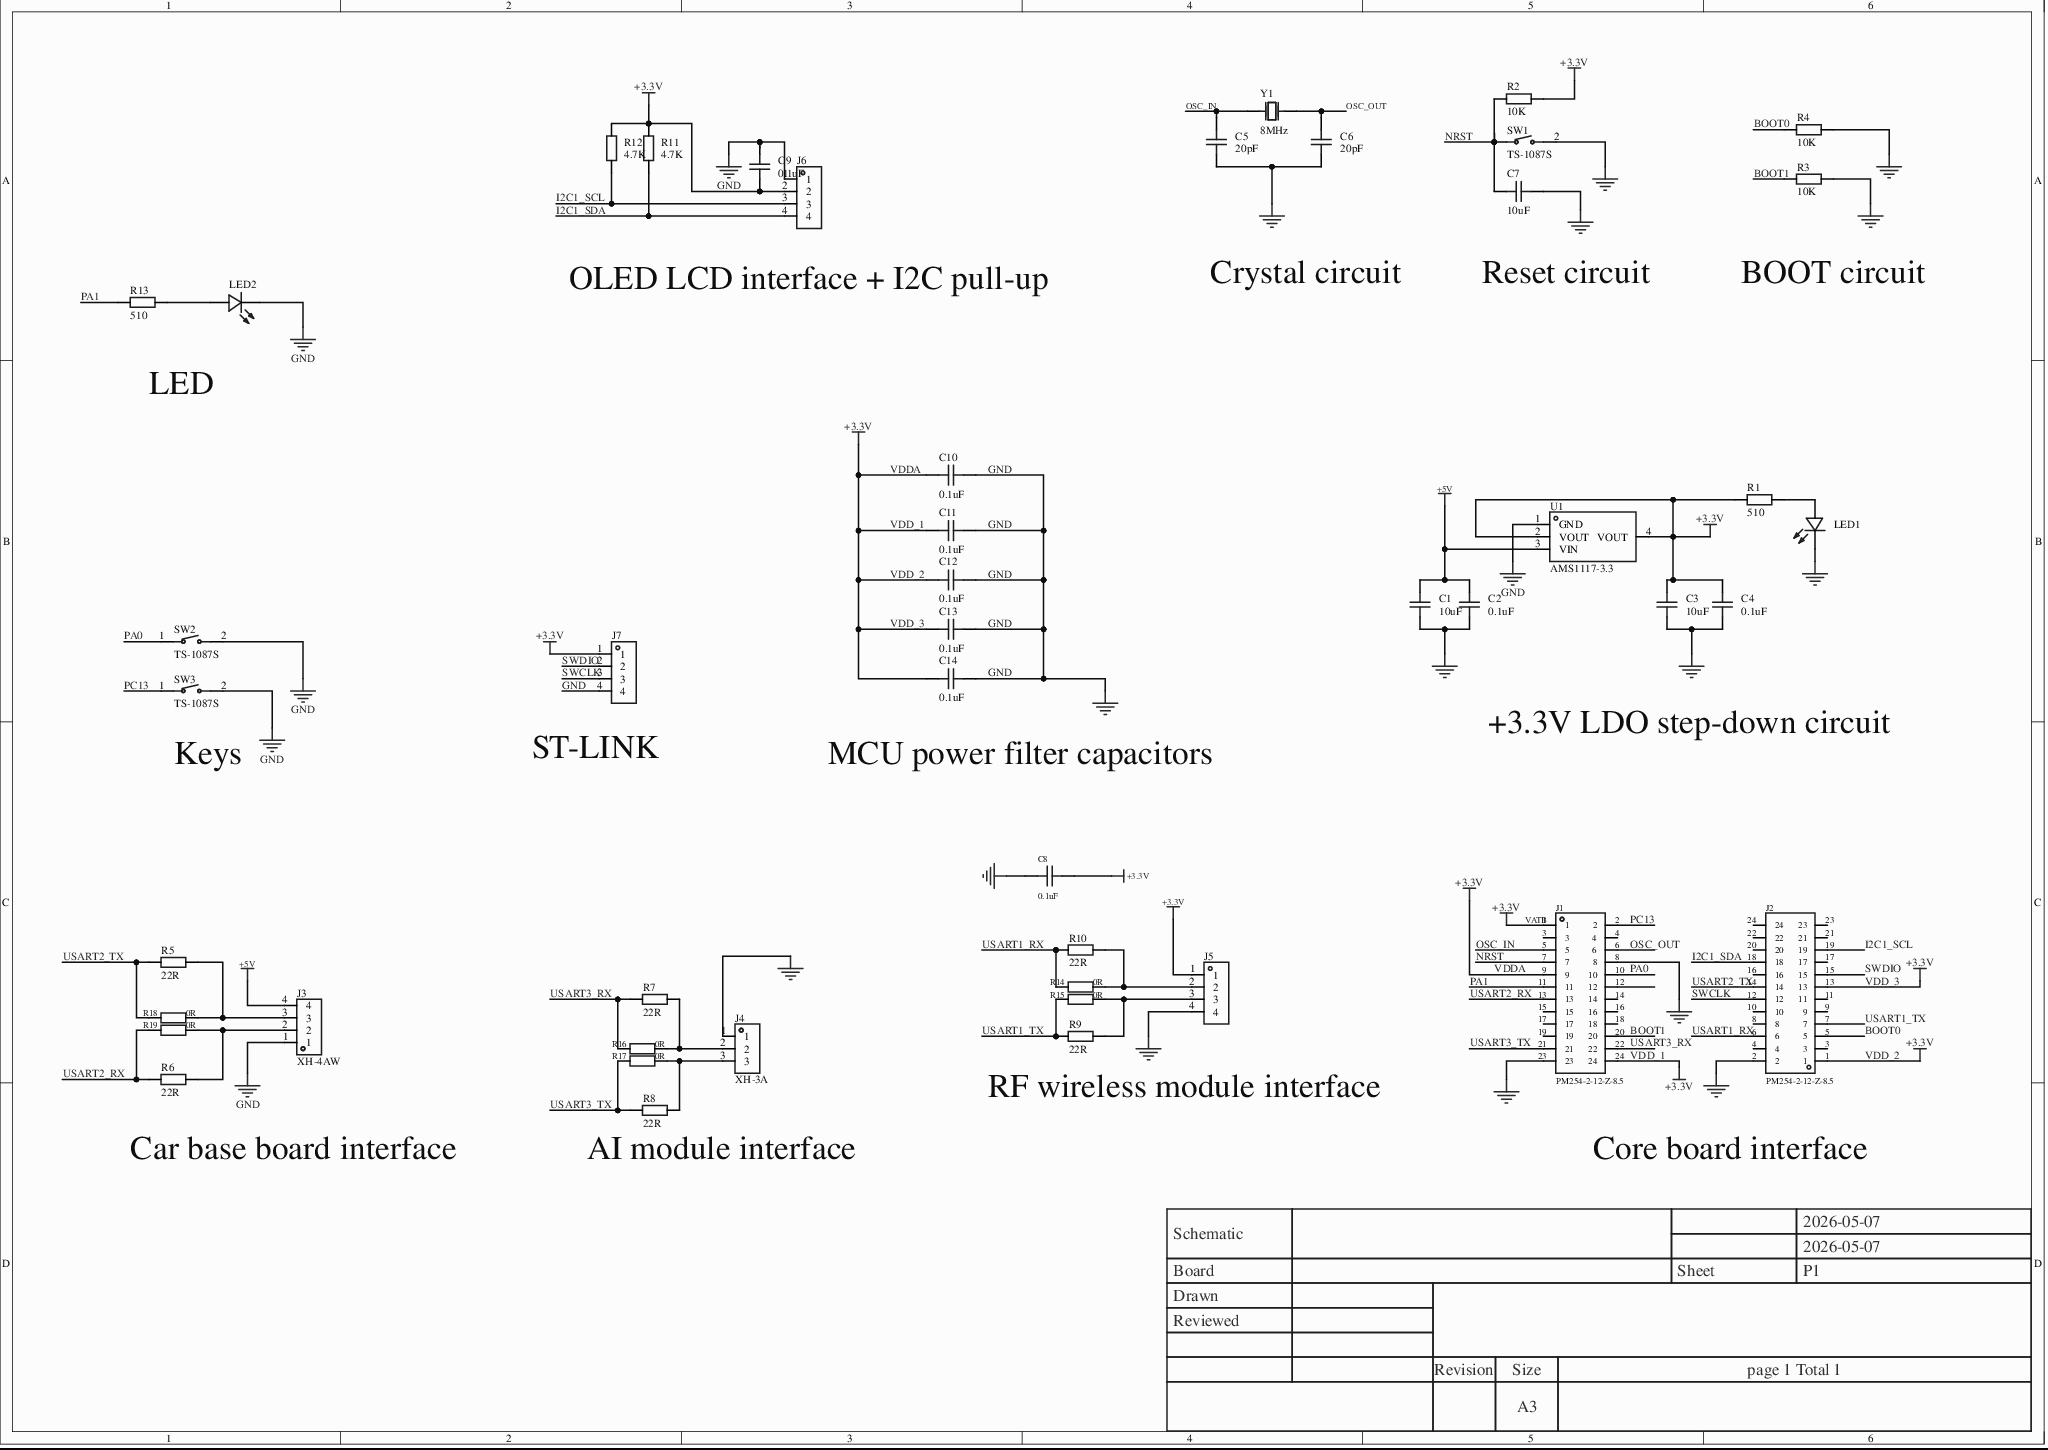
[diagram p0: MISC52078-3.schdoc]
# Altium project MISC52078-2.PrjPcb
1 sheet, 47 parts. Net scope: global (net labels, ports and power ports of the same name join across sheets).
Board file: MISC52078.pcbdoc

## Sheet MISC52078-3.schdoc
size 420 x 297 mm; Version: V1.0; @Project Name: MISC52078; @Update Date: 2026-05-23; @Create Date: 2026-05-23; @Board Name: MISC52078; @Create Time: 04:19:49; @Page Count: 1; @Page No: 1; @Schematic Name: MISC52078; @Update Time: 12:19:49; Size: A4

### Parts
C1  10uF  [C0805]
C2  0.1uF  [C0805]
C3  10uF  [C0805]
C4  0.1uF  [C0805]
C5  20pF  [C0805]
C6  20pF  [C0805]
C7  10uF  [C0805]
C8  0.1uF  [C0603]
C9  0.1uF  [C0805]
C10  0.1uF  [C0805]
C11  0.1uF  [C0805]
C12  0.1uF  [C0805]
C13  0.1uF  [C0805]
C14  0.1uF  [C0805]
J1  PM254-2-12-Z-8.5  [HDR-TH_24P-P2.54-V-F-R2-C12-S2.54-2]
J2  PM254-2-12-Z-8.5  [HDR-TH_24P-P2.54-V-F-R2-C12-S2.54-2]
J3  XH-4AW  [CONN-TH_XH-4AW]
J4  XH-3A  [CONN-TH_XH-3A]
J5  (no value)  [CONN-TH_4P-P2.54-L10.2-W2.5]
J6  (no value)  [CONN-TH_4P-P2.54-L10.2-W2.5]
J7  (no value)  [CONN-TH_4P-P2.54-L10.2-W2.5]
LED1  KT-0805W  [LED0805-R-RD]  (value not drawn)
LED2  (no value)  [LED0805-R-RD]
R1  510  [R0805]
R2  10K  [R0805]
R3  10K  [R0805]
R4  10K  [R0805]
R5  22R  [R0805]
R6  22R  [R0805]
R7  22R  [R0805]
R8  22R  [R0805]
R9  22R  [R0805]
R10  22R  [R0805]
R11  4.7K  [R0805]
R12  4.7K  [R0805]
R13  510  [R0805]
R14  0R  [R0603]
R15  0R  [R0603]
R16  0R  [R0603]
R17  0R  [R0603]
R18  0R  [R0603]
R19  0R  [R0603]
SW1  TS-1087S  [SW-SMD_L5.2-W5.2-P3.70-LS6.4]
SW2  TS-1087S  [SW-SMD_L5.2-W5.2-P3.70-LS6.4]
SW3  TS-1087S  [SW-SMD_L5.2-W5.2-P3.70-LS6.4]
U1  AMS1117-3.3  [SOT-223-3_L6.5-W3.4-P2.30-LS7.0-BR]
Y1  8MHz  [CRYSTAL-SMD_L11.5-W4.8-LS12.7]

### Nets
+5V: C1.1 C2.1 J3.4 U1.3(VIN)
GND: C1.2 C2.2 C3.1 C4.1 C5.1 C6.1 C7.2 C8.1 C9.2 C10.2 C11.2 C12.2 C13.2 C14.2 J1.8 J1.23 J2.2 J3.1 J4.1 J5.4 J6.1 J7.4 LED1.2(K) LED2.2(K) R3.2 R4.2 SW1.2 SW2.2 SW3.2 U1.1(GND)
+3.3V: C3.2 C4.2 C8.2 C9.1 C10.1 C11.1 C12.1 C13.1 C14.1 J1.1 J1.9 J1.24 J2.1 J2.13 J5.1 J6.2 J7.1 R1.1 R2.2 R11.2 R12.2 U1.2(VOUT) U1.4(VOUT)  [also labelled VATB, VDD_1, VDD_2, VDD_3, VDDA]
BOOT0: J2.5 R4.1
BOOT1: J1.20 R3.1
I2C1_SCL: J2.19 J6.3 R12.1
I2C1_SDA: J2.18 J6.4 R11.1
NRST: C7.1 J1.7 R2.1 SW1.1
OSC_IN: C5.2 J1.5 Y1.2(OSC2)
OSC_OUT: C6.2 J1.6 Y1.1(OSC1)
PA0: J1.10 SW2.1
PA1: J1.11 R13.1
PC13: J1.2 SW3.1
SWCLK: J2.12 J7.3
SWDIO: J2.15 J7.2
USART1_RX: J2.6 R10.1 R14.1
USART1_TX: J2.7 R9.1 R15.1
USART2_RX: J1.13 R6.1 R19.1
USART2_TX: J2.14 R5.1 R18.1
USART3_RX: J1.22 R7.1 R16.1
USART3_TX: J1.21 R8.1 R17.1
NetJ3_2: J3.2 R6.2 R19.2
NetJ3_3: J3.3 R5.2 R18.2
NetJ4_2: J4.2 R7.2 R16.2
NetJ4_3: J4.3 R8.2 R17.2
NetJ5_2: J5.2 R10.2 R14.2
NetJ5_3: J5.3 R9.2 R15.2
NetLED1_1: LED1.1(A) R1.2
NetLED2_1: LED2.1(A) R13.2

Not connected (* = marked no-connect by the designer): J1 3* 4* 12 14* 15* 16* 17* 18* 19*; J2 3* 4* 8* 9* 10* 11* 16* 17* 20* 21* 22* 23* 24*

### Notes on the sheet
- (near J6) OLED LCD interface + I2C pull-up
- Crystal circuit
- Reset circuit
- BOOT circuit
- LED
- (near SW3) Keys
- (near J7) ST-LINK
- MCU power filter capacitors
- +3.3V LDO step-down circuit
- (near R9) RF wireless module interface
- Car base board interface
- (near R8) AI module interface
- Core board interface
- 2026-05-07
- Schematic
- Board
- Sheet
- P1
- Drawn
- Reviewed
- Revision
- Size
- A3
- page 1 Total 1

### Library data of the parts
C1-C7 C9-C14 = CAP_0603: Symbol: Capacitance; ConvertToPcb: yes; ModelId: ac125912035d415993ca9572d50418b10819f05c4eef4c71ace90d822a990e87; ModelName: C0603_L1.6-W0.8-H0.8; ModelTransform: 62.992,31.496,0,0,0,0,0,0,0; Device: CAP_0603; FootprintName: C0805; AddInBom: yes; Supplier Footprint: 0603
  C1 C3 C7: Value: 10uF
  C2 C4 C9-C14: Value: 0.1uF
  C5 C6: Value: 20pF
C8 = CAP_0603: Symbol: CapAcitance; ConvertToPcb: yes; ModelId: ac125912035d415993ca9572d50418b10819f05c4eef4c71ace90d822a990e87; ModelName: C0603_L1.6-W0.8-H0.8; ModelTransform: 62.992,31.496,0,0,0,0,0,0,0; Device: CAP_0603; Value: 0.1uF; AddInBom: yes; Supplier Footprint: 0603; FootprintName: C0603
J1 J2 = PM254-2-12-Z-8.5: Manufacturer: HCTL(华灿天禄); Holes Structure: 2x12P; Pitch: 2.54mm; Circular Hole / Square Hole: Square hole; Number of Positions: 24P; Current Rating: 3A; Holes Direction: Top; 3D Model: 8679914d7755405889364377e1fa0432; 3D Model Transform: 1215.74568,196.85,0,0,0,0,0,0,-125.984; AddInBom: yes; Symbol: PM254-2-12-Z-8.5; Device: PM254-2-12-Z-8.5; LCSC Part Name: 2x12P 间距:2.54mm 直插; Supplier Part: C2897413; Manufacturer Part: PM254-2-12-Z-8.5; Supplier Footprint: 插件,P=2.54mm; JLCPCB Part Class: Extended library; Datasheet: https://example.com/datasheet/PM254-2-12-Z-8.5/3142418.html; Supplier: LCSC; Row Spacing: 2.54mm; Mounting Type: Through-hole; Number of Rows: Dual row; Voltage Rating (Max): -; Insulation Height: 8.5mm; Contact Material: Copper alloy; Operating Temperature: -40℃~+105℃; FootprintName: HDR-TH_24P-P2.54-V-F-R2-C12-S2.54-2; ConvertToPcb: yes; ModelName: HDR-TH_24P-P2.54-V-F-R2-C12-S2.54-2
J3 = XH-4AW: Manufacturer: HCTL(华灿天禄); Symbol: XH-4AW_C2908613; Pins Structure: 1x4P; Pitch: 2.54mm; Reference Series: XH; Number of PINs Per Row: 4; Current Rating: 3A; Voltage Rating: 250V; Plastic Material: PA66; Flame Retardant Rating: UL94V-0; Z-Height of the Board: 5.9mm; Y-Width of Bottom Edge on Board: 7mm; 3D Model: 82fee406c0fb42748bb7a39a83218b360819f05c4eef4c71ace90d822a990e87; 3D Model Transform: 492.125,303.936,0,0,0,0,-0.004,-139.091,-118.11; AddInBom: yes; Device: XH-4AW; LCSC Part Name: 1x4P 间距:2.54mm 弯插 系列:XH; Supplier Part: C2908613; Manufacturer Part: XH-4AW; Supplier Footprint: 弯插,P=2.5mm; JLCPCB Part Class: Extended Part; Datasheet: https://example.com/datasheet/XH-4AW/3184384.html; Supplier: LCSC; Mounting Type: Right-angle; Number of Pins: 4P; Number of Rows: 1; Row Spacing: -; Contact Material: Brass; Contact Plating: Tin; Operating Temperature: -25℃~+85℃; FootprintName: CONN-TH_XH-4AW; ConvertToPcb: yes; ModelName: CONN-TH_XH-4AW
J4 = XH-3A: Manufacturer: HCTL(华灿天禄); Symbol: XH-3A_C2908601; Pins Structure: 1x3P; Pitch: 2.5mm; Reference Series: XH; Number of PINs Per Row: 3; Current Rating: 3A; Voltage Rating: 250V; Plastic Material: PA66; Flame Retardant Rating: UL94V-0; Z-Height of the Board: 7mm; Y-Width of Bottom Edge on Board: 5.9mm; 3D Model: 37b0cc6608c7491e85fcc981bb0e57920819f05c4eef4c71ace90d822a990e87; 3D Model Transform: 393.7,224.44837,0,180,0,0,-0.005,17.716,-98.425; AddInBom: yes; ModelName: XH2.5-3A; Device: XH-3A; LCSC Part Name: 1x3P 间距:2.5mm 直插 系列:XH; Supplier Part: C2908601; Manufacturer Part: XH-3A; Supplier Footprint: 插件,P=2.5mm; JLCPCB Part Class: Extended Part; Datasheet: https://example.com/datasheet/XH-3A/3184372.html; Supplier: LCSC; Mounting Type: Through-hole; Number of Pins: 3P; Number of Rows: 1; Row Spacing: -; Contact Material: Brass; Contact Plating: Tin; Operating Temperature: -25℃~+85℃; FootprintName: CONN-TH_XH-3A; ConvertToPcb: yes
J5 = POGOPIN-4P-2.54-17.0H-2.0T: 3D Model: 8000fb388bc741e4ad891e3721997f230819f05c4eef4c71ace90d822a990e87; 3D Model Transform: 401.574,98.8187,0,0,0,0,0,0,-78.74; AddInBom: yes; Symbol: POGOPIN-4P-2.54-17.0H-2.0T; Device: POGOPIN-4P-2.54-17.0H-2.0T; LCSC Part Name: POGOPIN-4P-2.54-17.0H-2.0T; Supplier Part: C9900021787; Supplier Footprint: 4P-2.54-17.0H-2.0T; JLCPCB Part Class: Extended Part; Supplier: LCSC; FootprintName: CONN-TH_4P-P2.54-L10.2-W2.5; ConvertToPcb: yes; ModelName: CONN-TH_4P-P2.54-L10.2-W2.5
J6 J7 = POGOPIN-4P-2.54-17.0H-2.0T: AddInBom: yes; ModelId: 8000fb388bc741e4ad891e3721997f230819f05c4eef4c71ace90d822a990e87; ModelTransform: 401.574,98.8187,0,0,0,0,0,0,-78.74; Device: POGOPIN-4P-2.54-17.0H-2.0T; Symbol: POGOPIN-4P-2.54-17.0H-2.0T; FootprintName: CONN-TH_4P-P2.54-L10.2-W2.5; LCSC Part Name: POGOPIN-4P-2.54-17.0H-2.0T; SupplierPart: C9900021787; Supplier Footprint: 4P-2.54-17.0H-2.0T; JLCPCB Part Class: Extended Part; Supplier: LCSC; ConvertToPcb: yes; ModelName: CONN-TH_4P-P2.54-L10.2-W2.5
LED1 LED2 = KT-0805W: Manufacturer: KENTO; Symbol: whiteLEDSMD; AddInBom: yes; Illumination Color: White; Voltage - Forward(Vf): 2.6V~3.2V; Power(Watts): 80mW; Forward Current: 25mA; Diode Configuration: Independent diode; Lens Color: Yellow lens; Color Temperature: 13172K~100000K; Luminous Intensity: 350mcd; Viewing Angle: 120°; ModelId: 6ccd75a2b5134d6ab756ecf3c14a72900819f05c4eef4c71ace90d822a990e87; ModelName: LED0805-RD; ModelTransform: 79.527,49.2125,0,0,0,0,0,0,0; Device: KT-0805W; FootprintName: LED0805-R-RD; LCSC Part Name: 0805 白灯 高亮; SupplierPart: C34499; Supplier Footprint: 0805; JLCPCB Part Class: Basic Part; Datasheet: https://example.com/datasheet/KT-0805W/35468.html; Supplier: LCSC; ConvertToPcb: yes; Lamp Holder Type: -; Wavelength - Dominant: -; Peak Wavelength: -; Mounting Style: Top mount; Operating Temperature: -30℃~+85℃
  LED1: ManufacturerPart: KT-0805W
R1-R4 R11-R13 = Res_0603: Symbol: Resistor; ConvertToPcb: yes; ModelId: fc143cca1e79419f9cd78b61e9279f080819f05c4eef4c71ace90d822a990e87; ModelName: R0603; ModelTransform: 31.8897,63.7794,0,90,0,0,0,0,0; Device: Res_0603; FootprintName: R0805; AddInBom: yes; Supplier Footprint: 0603
  R1 R13: Value: 510
  R2-R4: Value: 10K
  R11 R12: Value: 4.7K
R5-R10 = Res_0603: Symbol: Resistor; 3D Model: fc143cca1e79419f9cd78b61e9279f080819f05c4eef4c71ace90d822a990e87; 3D Model Transform: 31.8897,63.7794,0,90,0,0,0,0,0; ConvertToPcb: yes; ModelName: R0603; Device: Res_0603; Value: 22R; Supplier Footprint: 0603; FootprintName: R0805; AddInBom: yes
R14 = Res_0603: Symbol: Resistor; ConvertToPcb: yes; ModelId: fc143cca1e79419f9cd78b61e9279f080819f05c4eef4c71ace90d822a990e87; ModelTransform: 31.8897,63.7794,0,90,0,0,0,0,0; Value: 10K; Device: Res_0603; AddInBom: yes; Supplier Footprint: 0603; FootprintName: R0603; ModelName: R0603
R15-R19 = Res_0603: Symbol: Resistor; ConvertToPcb: yes; ModelId: fc143cca1e79419f9cd78b61e9279f080819f05c4eef4c71ace90d822a990e87; ModelTransform: 31.8897,63.7794,0,90,0,0,0,0,0; Device: Res_0603; Value: 0R; AddInBom: yes; Supplier Footprint: 0603; FootprintName: R0603; ModelName: R0603
SW1-SW3 = TS-1087S-04026: Manufacturer: XUNPU(讯普); AddInBom: yes; Circuit: SPST; Actuator Style: Round button; Switch Length: 5.2mm; Switch Height: 4mm; Contact Current: 50mA; Voltage Rating (DC): 12V; ModelId: 81be6fddaf4346549e990750dca182690819f05c4eef4c71ace90d822a990e87; ModelName: SW-SMD_L5.2-W5.2-H4.5-P3.70-LS6.4; ModelTransform: 251.968,204.724,0,0,0,0,0,0,0; Device: TS-1087S-04026; Symbol: TS-1087S-04026; Manufacturer Part: TS-1087S; FootprintName: SW-SMD_L5.2-W5.2-P3.70-LS6.4; LCSC Part Name: 5.2*5.2*4mm 立贴 轻触开关; SupplierPart: C455272; Supplier Footprint: SMD,5.2x5.2mm; JLCPCB Part Class: Extended Part; Datasheet: https://example.com/upload/public/pdf/source/20191118/C455274_574AF48D0973B20F599903060160141E.pdf; Supplier: LCSC; ConvertToPcb: yes; Mounting Style: Vertical mount; Switch Width: 5.2mm; With Lamp: -; Mechanical Life: -
U1 = AMS1117-3.3_C6186: Manufacturer: AMS; AddInBom: yes; Output Type: Fixed; Voltage - Supply: 15V; Output Voltage: 3.3V; Output Current: 1A; Power Supply Rejection Ratio (PSRR): 72dB@(120Hz); Voltage Dropout: 1.1V@(800mA); standby current: 5mA; Noise: 0.003%Vout; Output Configuration: Positive; Number of Outputs: 1; ModelId: 925194bf9823436183a3e0b978a8d0760819f05c4eef4c71ace90d822a990e87; ModelName: SOT-223-4P_L6.5-W3.5-H1.6-LS7.0-P2.30; ModelTransform: 279.89794,255.905,0,180,0,0,-3.9385,-0.0005,0; Device: AMS1117-3.3_C6186; Symbol: AMS1117-3.3; FootprintName: SOT-223-3_L6.5-W3.4-P2.30-LS7.0-BR; LCSC Part Name: 3.3V 1A 15V; SupplierPart: C6186; ManufacturerPart: AMS1117-3.3; Supplier Footprint: SOT-223; JLCPCB Part Class: Basic Part; Datasheet: https://example.com/datasheet/AMS1117-3.3/6652.html; Supplier: LCSC; ConvertToPcb: yes; Features: Overcurrent protection; thermal shutdown; Operating Temperature: -40℃~+125℃
Y1 = X49SM8MSD2SC: Manufacturer: YXC(扬兴晶振); AddInBom: yes; Normal temperature Frequency Tolerance: ±20ppm; Load Capacitance: 20pF; Frequency Stability: ±30ppm; ModelId: 6f569b91267b44029b8615eb5c810fba0819f05c4eef4c71ace90d822a990e87; ModelName: HC-49S_L11.4-W1.8-H3.0-LS12.7; ModelTransform: 499.999,188.976,0,180,0,0,0.002,-0.002,0; Device: X49SM8MSD2SC; Symbol: X49SM8MSD2SC; FootprintName: CRYSTAL-SMD_L11.5-W4.8-LS12.7; LCSC Part Name: HC-49SMD 8MHZ 20PF ±20PPM -20~70℃（±30PPM）; SupplierPart: C12674; ManufacturerPart: X49SM8MSD2SC; Supplier Footprint: HC-49S-SMD; JLCPCB Part Class: Basic Part; Datasheet: https://example.com/datasheet/X49SM8MSD2SC/13310.html; Supplier: LCSC; ConvertToPcb: yes; Type: SMD crystal; Value: 8MHz; Operating Temperature: -20℃~+70℃